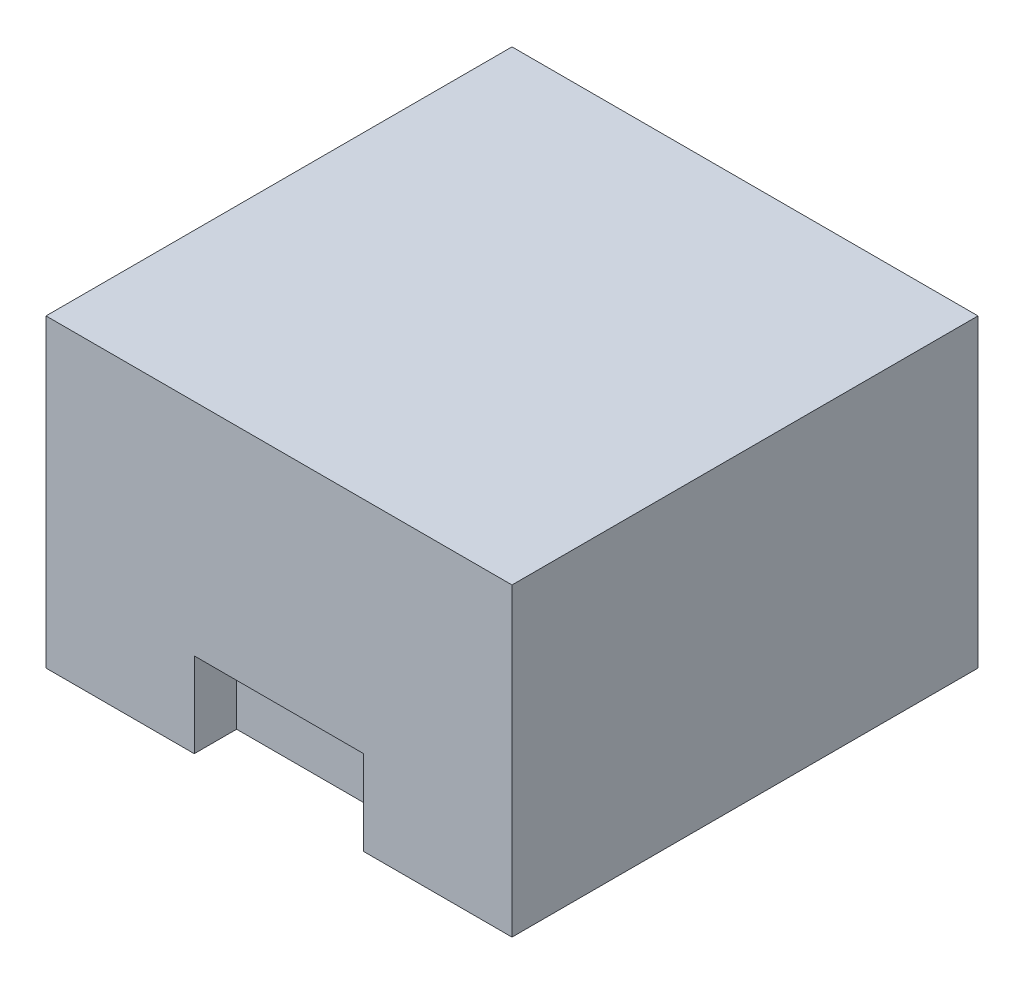
from build123d import *

# Parameters (mm, degrees)
SKETCH1_W           = 110
SKETCH1_H           = 110
BOSS_EXTRUDE1_DEPTH = 72
SKETCH2_W           = 40
SKETCH2_H           = 20
CUT_EXTRUDE1_DEPTH  = 10


with BuildPart() as part:
    # Sketch1 → Boss-Extrude1 (new body)
    with BuildSketch(Plane(origin=(0, 0, 0), x_dir=(1, 0, 0), z_dir=(0, 1, 0))):
        Rectangle(SKETCH1_W, SKETCH1_H)
    extrude(amount=BOSS_EXTRUDE1_DEPTH)

    # Sketch2 → Cut-Extrude1 (cut)
    with BuildSketch(Plane.XY.offset(55)):
        with Locations((0, 10)):
            Rectangle(SKETCH2_W, SKETCH2_H)
    extrude(amount=-CUT_EXTRUDE1_DEPTH, mode=Mode.SUBTRACT)


solid = part.part
